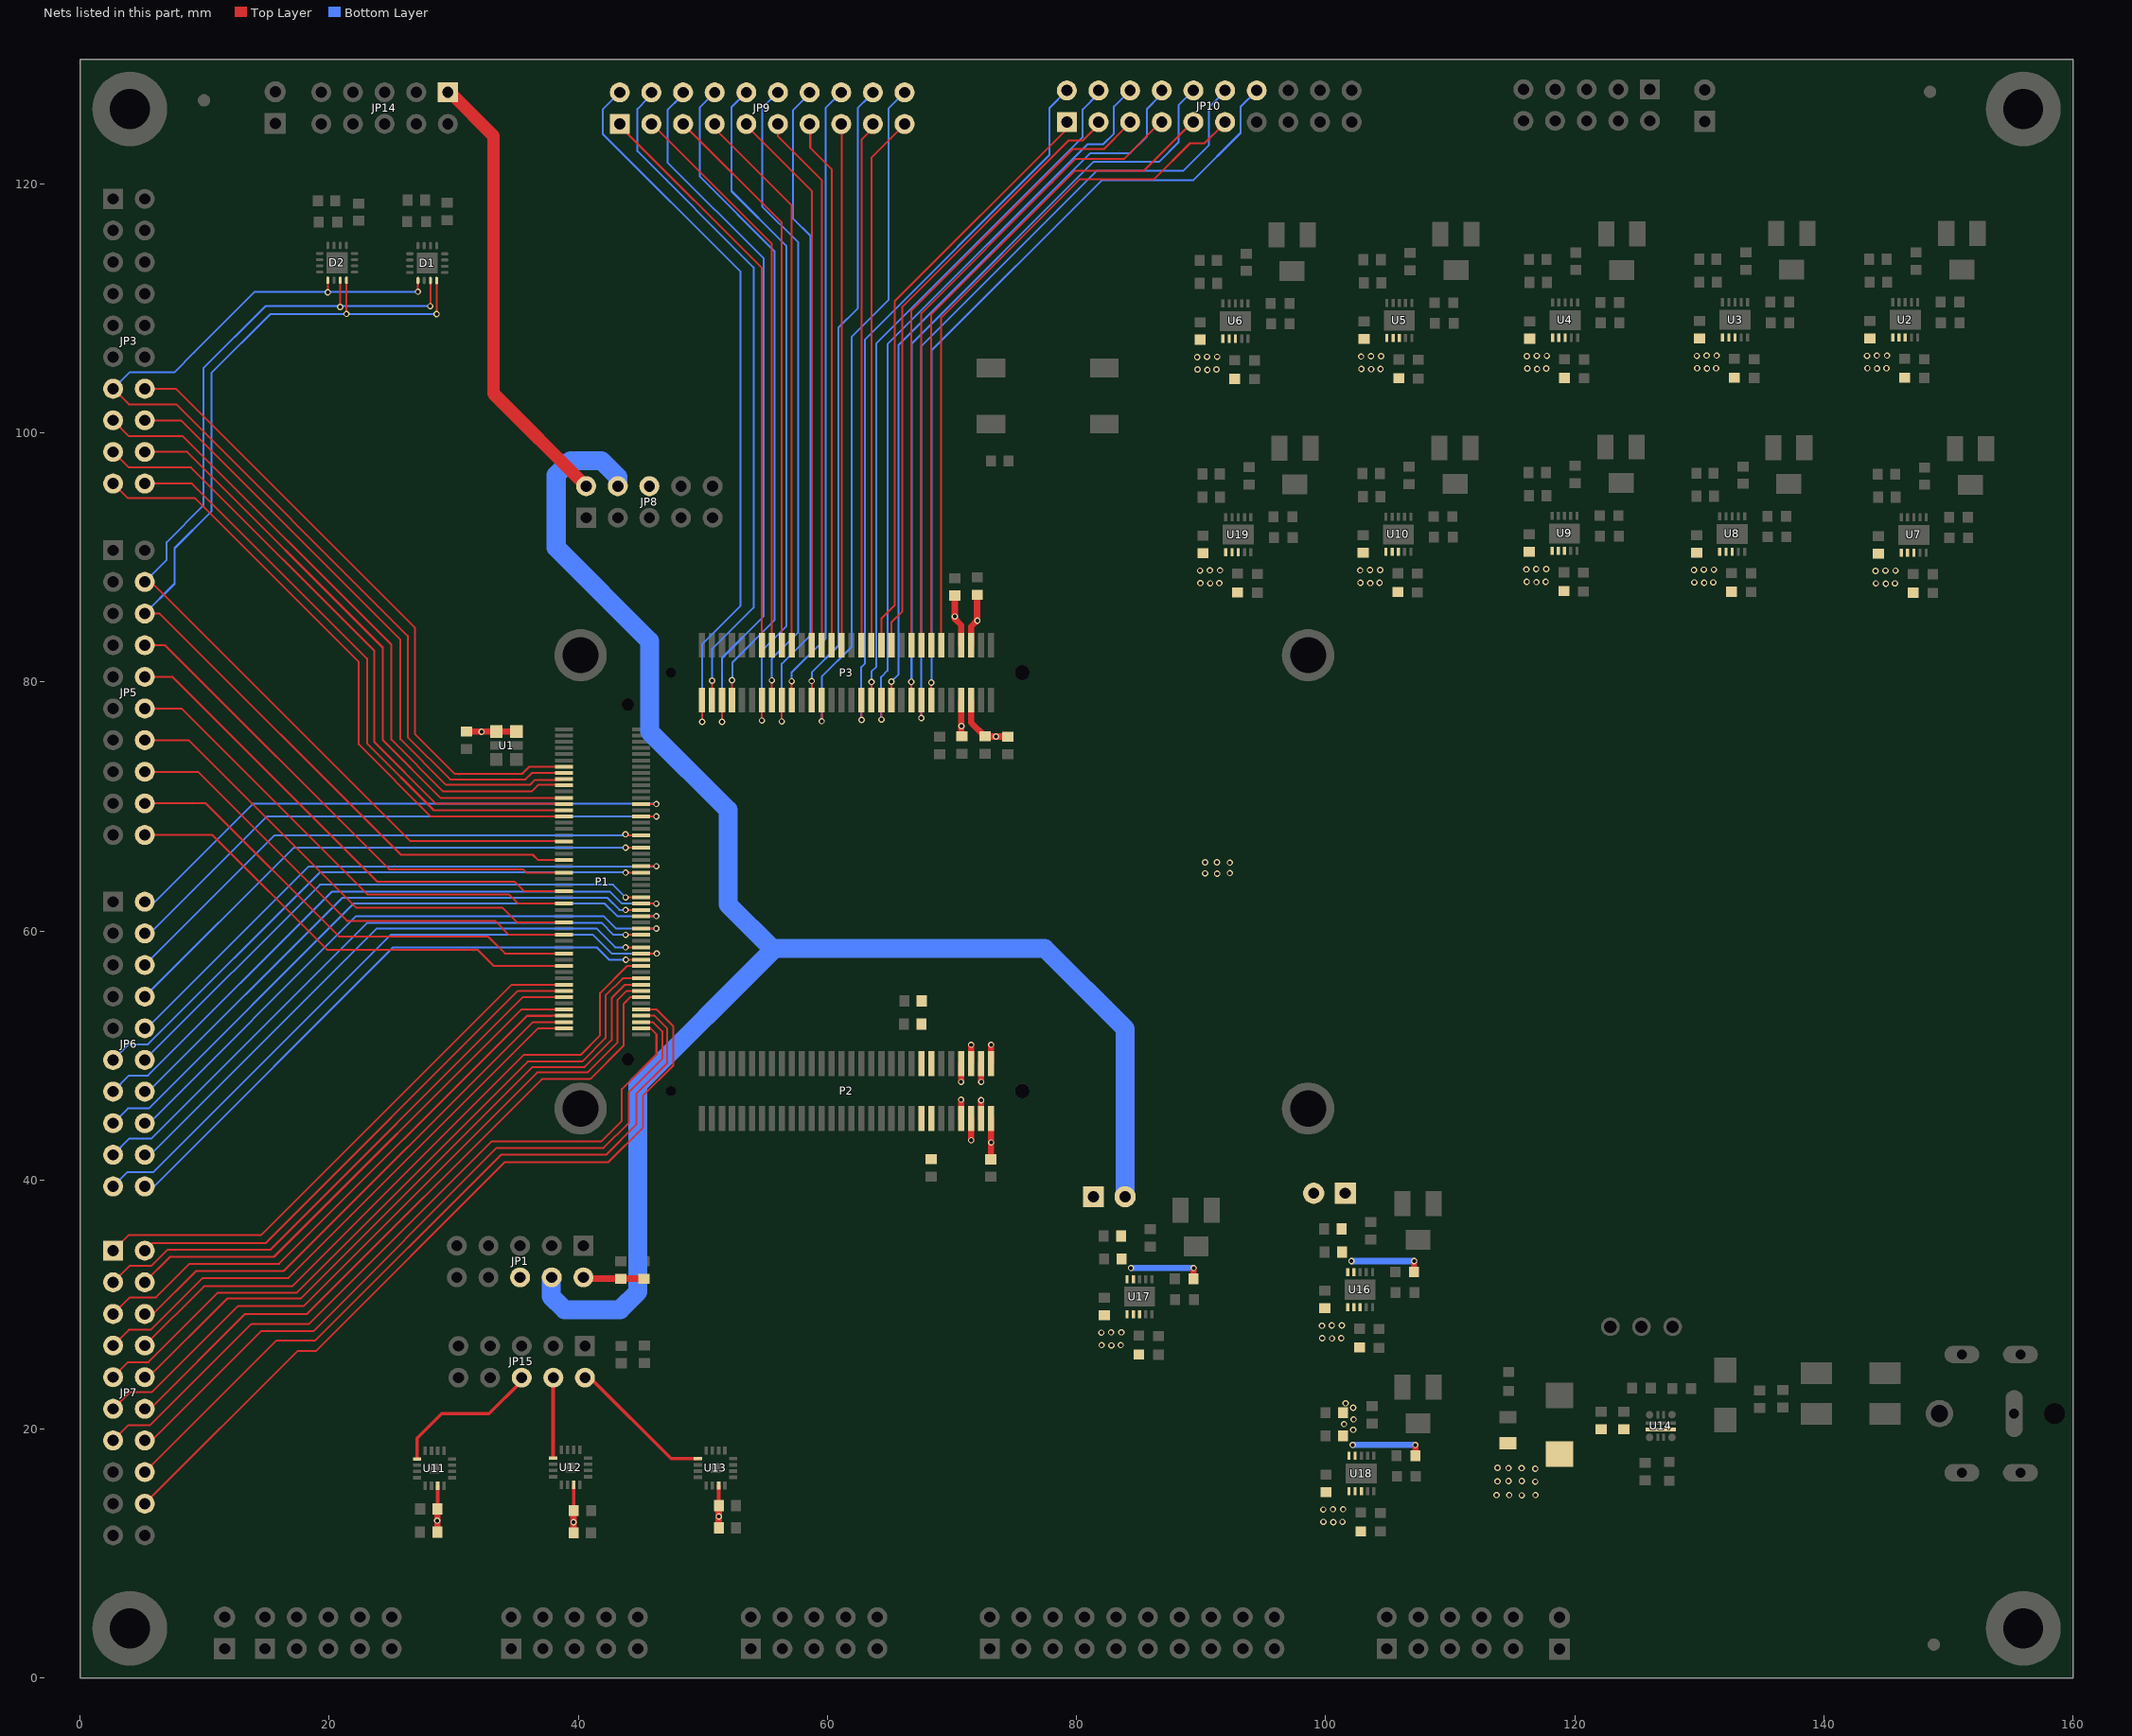
[diagram p0: the nets of this part, all layers, seen from the top]
# Altium PCB MISC82195.PcbDoc (part 6 of 8)
Units mm, origin at the board's own origin, x right, y up, seen from the top; angles counter-clockwise.
Board outline 160 x 130 mm, 4 copper layers (Top Layer, GND, POWER, Bottom Layer); 214 components, 251 nets, 1068 pads, 1218 vias.

## Via types
v1: diameter 0.508, hole 0.305, Top Layer to Bottom Layer, 1218 vias

## Nets (pads, with @x,y where several pads share a name; then routed paths per layer and width w, separated by ;. In a path a pad name is that pad's centre, name@x,y a point inside that pad or via, vN(x,y) a via of type N, cw(c..) or ccw(c..) an arc to the next point about the centre after c; other vN are vias at no path point) (continued)
PW53: JP6.11 P1.B47 | length 48.8
  Top Layer w0.152: v1(43.803,64.688) P1.B47@45.038,64.688
  Bottom Layer w0.152: JP6.11@2.658,49.642 3.918,50.902 5.461,50.902 19.253,64.694 v1@43.965,64.694
PW54: JP6.13 P1.B57 | length 51.9
  Top Layer w0.152: P1.B57@45.038,62.188 v1(46.274,62.188)
  Bottom Layer w0.152: JP6.13@2.658,47.102 3.943,48.387 5.461,48.387 20.244,63.17 42.52,63.17 43.501,62.188 v1(46.274,62.188)
PW55: JP6.15 P1.B61 | length 52.6
  Top Layer w0.152: P1.B61@45.038,61.188 v1(46.274,61.188)
  Bottom Layer w0.152: JP6.15@2.658,44.562 3.841,45.745 5.512,45.745 21.971,62.205 42.113,62.205 43.129,61.188 v1(46.274,61.188)
PW56: JP6.17 P1.B67 | length 50.5
  Top Layer w0.152: v1(43.803,59.688) P1.B67@45.038,59.688
  Bottom Layer w0.152: JP6.17@2.658,42.022 3.968,43.332 5.74,43.332 23.063,60.655 41.859,60.655 42.826,59.688 v1(43.803,59.688)
PW57: JP6.19 P1.B73 | length 53.9
  Top Layer w0.152: P1.B73@45.038,58.188 v1(46.301,58.188)
  Bottom Layer w0.152: JP6.19@2.658,39.482 3.816,40.64 5.893,40.64 24.968,59.715 41.148,59.715 42.672,58.191 46.298,58.191 v1(46.301,58.188)
PW58: JP7.1 P1.B84 | length 45.1
  Top Layer w0.152: JP7.1@2.658,34.326 3.892,35.56 14.529,35.56 34.657,55.688 P1.B84@38.866,55.688
PW59: JP7.3 P1.B88 | length 45.7
  Top Layer w0.152: JP7.3@2.658,31.786 3.968,33.096 5.715,33.096 7.01,34.392 15.265,34.392 35.562,54.688 P1.B88@38.866,54.688
PW60: JP7.5 P1.B94 | length 48.2
  Top Layer w0.152: JP7.5@2.658,29.246 3.994,30.582 6.096,30.582 8.788,33.274 15.977,33.274 35.865,53.162 ; 37.914,53.162 35.865,53.162 ; P1.B94@38.866,53.188 35.891,53.188 35.865,53.162
PW61: JP7.7 P1.B98 | length 46.8
  Top Layer w0.152: JP7.7@2.658,26.706 3.918,27.965 5.69,27.965 9.855,32.131 16.739,32.131 36.796,52.188 P1.B98@38.866,52.188
PW62: JP7.9 P1.B81 | length 58.7
  Top Layer w0.152: JP7.9@2.658,24.166 3.867,25.375 5.486,25.375 11.074,30.963 17.399,30.963 35.941,49.505 40.31,49.505 42.189,51.384 42.189,53.797 ; 42.189,54.331 42.189,53.797 ; 44.086,56.185 43.561,56.185 ; P1.B81@45.038,56.188 43.565,56.188 43.561,56.185 ; 42.189,53.797 42.189,54.813 43.536,56.159 43.561,56.185
PW63: JP7.11 P1.B85 | length 58.3
  Top Layer w0.152: JP7.11@2.658,21.626 3.994,22.962 5.766,22.962 12.675,29.87 17.932,29.87 36.703,48.641 40.742,48.641 43.129,51.029 43.129,54.432 43.885,55.188 P1.B85@45.038,55.188
PW64: JP7.13 P1.B97 | length 61
  Top Layer w0.152: JP7.13@2.658,19.086 3.867,20.295 5.613,20.295 13.767,28.448 18.39,28.448 33.045,43.104 41.859,43.104 43.497,44.742 43.497,47.307 46.279,50.089 46.279,51.689 45.771,52.197 P1.B97@45.441,52.197 ; P1.B97@45.038,52.188 P1.B97@45.441,52.188
PW65: JP7.18 P1.B91 | length 64.8
  Top Layer w0.152: JP7.18@5.198,14.006 17.456,26.264 18.923,26.264 34.087,41.427 42.418,41.427 45.212,44.221 45.212,46.787 47.625,49.2 47.625,52.349 46.279,53.696 P1.B91@45.491,53.696 ; P1.B91@45.038,53.688 P1.B91@45.491,53.688
PW66: JP7.16 P1.B93 | length 62.3
  Top Layer w0.152: JP7.16@5.198,16.546 15.754,27.102 18.872,27.102 33.807,42.037 42.24,42.037 44.653,44.45 44.653,46.914 47.142,49.403 47.142,52.172 46.126,53.188 P1.B93@45.415,53.188 ; P1.B93@45.038,53.188 P1.B93@45.415,53.188
PW67: JP7.14 P1.B95 | length 59.9
  Top Layer w0.152: JP7.14@5.198,19.086 5.751,19.086 14.529,27.864 18.745,27.864 33.452,42.57 42.037,42.57 44.069,44.602 44.069,47.066 46.736,49.733 46.736,51.867 46.736,51.943 45.991,52.688 P1.B95@45.038,52.688
PW68: JP7.12 P1.B87 | length 55.7
  Top Layer w0.152: JP7.12@5.198,21.626 5.624,21.626 13.233,29.235 18.212,29.235 37.084,48.108 40.97,48.108 43.637,50.775 43.637,53.01 ; 43.637,53.213 43.637,53.01 ; P1.B87@44.577,54.686 44.196,54.686 43.637,54.127 43.637,53.01 ; P1.B87@44.577,54.688 P1.B87@45.038,54.688
PW69: JP7.10 P1.B83 | length 55.5
  Top Layer w0.152: JP7.10@5.198,24.166 5.497,24.166 11.811,30.48 17.729,30.48 36.322,49.073 40.513,49.073 42.672,51.232 42.672,53.772 ; 42.672,54.077 42.672,53.772 ; 44.086,55.677 43.739,55.677 ; P1.B83@45.038,55.688 43.75,55.688 43.739,55.677 ; 42.672,53.772 42.672,54.61 43.713,55.651 43.739,55.677
PW70: JP7.8 P1.B77 | length 55
  Top Layer w0.152: JP7.8@5.198,26.706 9.963,31.471 17.043,31.471 35.611,50.038 40.183,50.038 41.758,51.613 41.758,54 ; 41.758,54.508 41.758,54 ; P1.B77@45.038,57.188 43.93,57.188 41.758,55.016 41.758,54
PW71: JP7.6 P1.B96 | length 43.4
  Top Layer w0.152: JP7.6@5.198,29.246 5.878,29.246 9.322,32.69 16.358,32.69 36.356,52.688 P1.B96@38.866,52.688
PW72: JP7.4 P1.B92 | length 42.7
  Top Layer w0.152: JP7.4@5.198,31.786 7.245,33.833 15.57,33.833 35.426,53.688 P1.B92@38.866,53.688
PW73: JP7.2 P1.B86 | length 42.3
  Top Layer w0.152: JP7.2@5.198,34.326 5.797,34.925 14.884,34.925 35.148,55.188 P1.B86@38.866,55.188
PW74: JP6.20 P1.B75 | length 48.2
  Top Layer w0.152: v1(43.82,57.688) P1.B75@45.038,57.688
  Bottom Layer w0.152: JP6.20@5.198,39.482 5.928,39.482 25.121,58.674 41.478,58.674 42.464,57.688 v1(43.82,57.688)
PW75: JP6.18 P1.B71 | length 48
  Top Layer w0.152: v1(43.804,58.688) P1.B71@45.038,58.688
  Bottom Layer w0.152: JP6.18@5.198,42.022 5.649,42.022 23.8,60.173 41.478,60.173 42.962,58.688 v1(43.804,58.688)
PW76: JP6.16 P1.B65 | length 49.6
  Top Layer w0.152: P1.B65@45.038,60.188 v1(46.274,60.188)
  Bottom Layer w0.152: JP6.16@5.198,44.562 5.547,44.562 22.174,61.189 42.037,61.189 43.037,60.188 v1(46.274,60.188)
PW77: JP6.14 P1.B59 | length 46.7
  Top Layer w0.152: v1(43.803,61.688) P1.B59@45.038,61.688
  Bottom Layer w0.152: JP6.14@5.198,47.102 5.497,47.102 21.057,62.662 42.342,62.662 43.315,61.688 v1(43.803,61.688)
PW78: JP6.12 P1.B55 | length 46.1
  Top Layer w0.152: v1(43.803,62.688) P1.B55@45.038,62.688
  Bottom Layer w0.152: JP6.12@5.198,49.642 19.262,63.706 42.786,63.706 v1(43.803,62.688)
PW79: JP6.10 P1.B45 | length 47.7
  Top Layer w0.152: P1.B45@45.038,65.188 v1(46.274,65.188)
  Bottom Layer w0.152: JP6.10@5.198,52.182 5.37,52.182 18.364,65.176 v1@46.262,65.176
PW80: JP6.8 P1.B39 | length 44.8
  Top Layer w0.152: v1(43.803,66.688) P1.B39@45.038,66.688
  Bottom Layer w0.152: JP6.8@5.198,54.722 17.176,66.7 v1@43.79,66.7
PW81: JP6.6 P1.B35 | length 44.3
  Top Layer w0.152: v1(43.79,67.767) 43.79,67.702 43.803,67.688 P1.B35@45.038,67.688
  Bottom Layer w0.152: JP6.6@5.198,57.262 15.627,67.691 v1@43.815,67.691
PW82: JP6.4 P1.B29 | length 46.2
  Top Layer w0.152: P1.B29@45.038,69.188 v1(46.274,69.188)
  Bottom Layer w0.152: JP6.4@5.198,59.802 5.598,59.802 14.986,69.19 46.273,69.19 v1(46.274,69.188)
PW83: JP6.2 P1.B25 | length 46
  Top Layer w0.152: P1.B25@45.038,70.188 v1(46.274,70.188)
  Bottom Layer w0.152: JP6.2@5.198,62.342 6.03,62.342 13.894,70.206 43.485,70.206 ; 43.891,70.206 43.485,70.206 ; v1(46.274,70.188) 46.257,70.206 43.485,70.206
PW84: JP5.20 P1.B78 | length 38
  Top Layer w0.152: JP5.20@5.198,67.701 10.632,67.701 19.837,58.496 31.902,58.496 33.21,57.188 P1.B78@38.866,57.188
PW85: JP5.18 P1.B74 | length 38.3
  Top Layer w0.152: JP5.18@5.198,70.241 10.099,70.241 20.777,59.563 32.741,59.563 34.112,58.191 P1.B74@38.506,58.191
PW86: JP5.16 P1.B68 | length 38.7
  Top Layer w0.152: JP5.16@5.198,72.781 9.464,72.781 21.438,60.808 33.325,60.808 34.442,59.69 P1.B68@38.481,59.69
PW87: JP5.14 P1.B64 | length 39.7
  Top Layer w0.152: JP5.14@5.198,75.321 8.727,75.321 22.174,61.874 33.909,61.874 35.103,60.681 P1.B64@38.837,60.681
PW88: JP5.12 P1.B58 | length 40.2
  Top Layer w0.152: JP5.12@5.198,77.861 8.143,77.861 23.063,62.941 34.442,62.941 35.195,62.188 P1.B58@38.866,62.188
PW89: JP5.10 P1.B54 | length 40.8
  Top Layer w0.152: JP5.10@5.198,80.401 7.407,80.401 23.851,63.957 34.9,63.957 35.668,63.188 P1.B54@38.866,63.188
PW90: JP5.8 P1.B48 | length 41.2
  Top Layer w0.152: JP5.8@5.198,82.941 6.822,82.941 24.816,64.948 35.56,64.948 35.819,64.688 P1.B48@38.866,64.688
PW91: D1.8 D2.8 JP5.6 P1.B44 | length 88.7
  Top Layer w0.152: JP5.6@5.198,85.481 6.391,85.481 25.756,66.116 36.347,66.116 36.775,65.688 P1.B44@38.866,65.688 ; v1(21.391,109.546) D2.8@21.391,112.25 ; v1@28.63,109.707 D1.8@28.63,112.224
  Bottom Layer w0.152: JP5.6@5.198,85.481 7.595,87.878 7.595,90.729 10.566,93.701 10.566,104.826 15.265,109.525 v1(28.626,109.525)
PW92: D1.7 D2.7 JP5.4 P1.B38 | length 86.2
  Top Layer w0.152: JP5.4@5.198,88.021 5.73,88.021 26.543,67.208 37.262,67.208 ; v1(20.891,110.096) D2.7@20.891,112.25 ; v1@28.13,110.248 D1.7@28.13,112.224 ; 37.897,67.208 37.262,67.208 ; P1.B38@38.608,67.208 37.262,67.208
  Bottom Layer w0.152: JP5.4@5.198,88.021 6.96,89.783 6.96,89.916 6.96,91.211 9.906,94.158 9.906,105.181 14.884,110.16 v1(28.118,110.16)
PW94: D1.5 D2.5 JP3.13 P1.B16 | length 83.7
  Top Layer w0.152: JP3.13@2.658,103.541 3.913,102.286 7.722,102.286 26.314,83.693 26.314,75.565 29.718,72.161 35.763,72.161 36.29,72.688 P1.B16@38.866,72.688 ; v1(19.891,111.28) D2.5@19.891,112.25 ; v1@27.13,111.407 D1.5@27.13,112.224
  Bottom Layer w0.152: JP3.13@2.658,103.541 3.968,104.851 7.569,104.851 9.182,106.464 14.046,111.328 v1(27.127,111.328)
PW95: JP3.14 P1.B14 | length 51.7
  Top Layer w0.152: JP3.14@5.198,103.541 7.686,103.541 26.873,84.353 26.873,75.819 30.074,72.619 35.509,72.619 36.079,73.188 P1.B14@38.866,73.188
PW96: JP3.15 P1.B20 | length 52.7
  Top Layer w0.152: JP3.15@2.658,101.001 3.938,99.72 8.255,99.72 24.994,82.982 24.994,75.362 29.159,71.196 36.246,71.196 36.779,71.73 P1.B20@38.354,71.73
PW97: JP3.16 P1.B18 | length 50.4
  Top Layer w0.152: JP3.16@5.198,101.001 8.118,101.001 25.73,83.388 25.73,75.387 29.388,71.73 36.119,71.73 36.525,72.136 P1.B18@38.608,72.136
PW98: JP3.17 P1.B26 | length 52.3
  Top Layer w0.152: JP3.17@2.658,98.461 3.913,97.206 8.915,97.206 23.622,82.499 23.622,75.159 28.575,70.206 37.592,70.206 ; 37.914,70.206 37.592,70.206 ; P1.B26@38.583,70.206 37.592,70.206
PW99: JP3.18 P1.B24 | length 49.1
  Top Layer w0.152: JP3.18@5.198,98.461 8.6,98.461 24.308,82.753 24.308,75.311 28.956,70.663 P1.B24@38.405,70.663
PW100: JP3.19 P1.B30 | length 50.9
  Top Layer w0.152: JP3.19@2.658,95.921 3.836,94.742 9.246,94.742 22.377,81.61 22.377,74.981 28.169,69.19 37.668,69.19 ; 37.871,69.19 37.668,69.19 ; P1.B30@38.43,69.19 37.668,69.19
PW101: JP3.20 P1.B28 | length 48.5
  Top Layer w0.152: JP3.20@5.198,95.921 8.981,95.921 23.038,81.864 23.038,75.057 28.406,69.688 P1.B28@38.866,69.688
PW102: JP9.1 P3.C13 | length 45.5
  Top Layer w0.152: JP9.1@43.967,124.003 54.737,113.233 P3.C13@54.737,82.939
PW103: JP9.3 P3.C15 | length 45.1
  Top Layer w0.152: JP9.3@46.431,124.282 55.537,115.176 P3.C15@55.537,82.939
PW104: JP9.5 P3.C17 | length 44.7
  Top Layer w0.152: JP9.5@48.692,124.511 56.337,116.865 P3.C17@56.337,82.939
PW105: JP9.7 P3.C19 | length 43.7
  Top Layer w0.152: JP9.7@51.181,124.206 57.137,118.25 P3.C19@57.137,82.939
PW106: JP9.9 P3.C23 | length 43.4
  Top Layer w0.152: JP9.9@53.873,124.282 58.737,119.418 P3.C23@58.737,82.939
PW107: JP9.11 P3.C25 | length 42.9
  Top Layer w0.152: JP9.11@56.007,124.384 56.007,123.825 59.537,120.295 P3.C25@59.537,82.939
PW108: JP9.13 P3.C27 | length 42.2
  Top Layer w0.152: JP9.13@58.623,124.409 58.623,122.885 60.337,121.171 P3.C27@60.337,82.939
PW109: JP9.15 P3.C29 | length 41.4
  Top Layer w0.152: P3.C29@61.137,82.939 JP9.15@61.137,124.359
PW110: JP9.17 P3.C33 | length 42
  Top Layer w0.152: P3.C33@62.737,82.939 62.737,123.52 JP9.17@63.754,124.536
PW111: JP9.19 P3.C35 | length 42.7
  Top Layer w0.152: P3.C35@63.537,82.939 63.537,122.084 JP9.19@66.04,124.587
PW112: JP10.1 P3.C37 | length 47.6
  Top Layer w0.152: P3.C37@64.337,82.939 64.337,85.089 65.405,86.157 65.405,110.566 JP10.1@79.248,124.409
PW113: JP10.3 P3.C39 | length 49.2
  Top Layer w0.152: P3.C39@65.137,82.939 65.137,84.797 66.015,85.674 66.015,110.134 79.35,123.469 80.493,123.469 JP10.3@81.661,124.638
PW114: JP10.5 P3.C43 | length 50.2
  Top Layer w0.152: P3.C43@66.737,82.939 66.737,109.816 77.673,120.752 77.749,120.828 79.705,122.784 82.22,122.784 JP10.5@83.972,124.536
PW115: JP10.7 P3.C45 | length 51.3
  Top Layer w0.152: P3.C45@67.539,83.617 67.539,109.601 78.003,120.066 78.08,120.142 79.908,121.971 83.795,121.971 JP10.7@86.589,124.765
PW116: JP10.9 P3.C47 | length 53.8
  Top Layer w0.152: P3.C47@68.337,82.939 68.337,109.511 79.883,121.056 85.42,121.056 JP10.9@89.027,124.663 ; JP10.9@89.052,124.638 JP10.9@89.205,124.79
PW117: JP10.11 P3.C49 | length 54.6
  Top Layer w0.152: P3.C49@69.139,83.566 69.139,109.245 80.264,120.371 86.233,120.371 89.103,123.241 90.272,123.241 JP10.11@91.669,124.638 ; JP10.11@91.707,124.6 JP10.11@91.745,124.638
PW118: JP10.14 P3.C48 | length 64
  Top Layer w0.152: P3.C48@68.337,78.539 v1(68.337,79.945)
  Bottom Layer w0.152: v1@68.351,80.01 68.351,106.604 82.017,120.269 89.357,120.269 93.167,124.079 93.167,126.187 JP10.14@94.463,127.483
PW119: JP10.12 P3.C46 | length 65.7
  Top Layer w0.152: v1(67.537,77.09) P3.C46@67.537,78.539
  Bottom Layer w0.152: v1(67.537,77.09) 67.537,106.958 81.61,121.031 88.544,121.031 90.627,123.114 90.627,126.136 JP10.12@91.745,127.254
PW120: JP10.10 P3.C44 | length 61.3
  Top Layer w0.152: P3.C44@66.737,78.539 v1(66.737,79.998)
  Bottom Layer w0.152: v1@66.751,80.086 66.751,107.137 81.382,121.768 86.639,121.768 88.189,123.317 88.189,126.289 JP10.10@89.383,127.483
PW121: JP10.8 P3.C40 | length 59.3
  Top Layer w0.152: P3.C40@65.137,78.539 v1(65.137,80.022)
  Bottom Layer w0.152: v1(65.137,80.022) 65.71,80.594 65.71,107.061 81.102,122.453 84.303,122.453 85.649,123.8 85.649,126.009 JP10.8@86.69,127.051
PW122: JP10.6 P3.C38 | length 61
  Top Layer w0.152: v1(64.337,76.961) P3.C38@64.337,78.539
  Bottom Layer w0.152: v1@64.313,77.089 64.313,80.391 64.821,80.899 64.821,107.112 80.874,123.165 82.144,123.165 83.007,124.028 83.007,126.187 JP10.6@84.303,127.483
PW123: JP10.4 P3.C36 | length 56.1
  Top Layer w0.152: P3.C36@63.537,78.539 v1(63.537,79.997)
  Bottom Layer w0.152: v1(63.537,79.997) 63.537,80.835 63.932,81.229 63.932,107.188 80.493,123.749 80.493,125.959 JP10.4@81.686,127.152
PW124: JP10.2 P3.C34 | length 58.8
  Top Layer w0.152: v1(62.737,76.937) P3.C34@62.737,78.539
  Bottom Layer w0.152: v1@62.713,77.089 62.713,81.178 63.017,81.483 63.017,107.493 77.826,122.301 77.826,126.086 JP10.2@79.223,127.483
PW125: JP9.20 P3.C26 | length 54.8
  Top Layer w0.152: v1(59.537,76.835) P3.C26@59.537,78.539
  Bottom Layer w0.152: v1@59.563,76.962 59.563,80.442 61.951,82.829 61.951,107.721 64.922,110.693 64.922,126.06 JP9.20@66.192,127.33
PW126: JP9.18 P3.C24 | length 50.3
  Top Layer w0.152: P3.C24@58.737,78.539 v1(58.737,80.073)
  Bottom Layer w0.152: v1(58.737,80.073) 58.737,80.759 60.884,82.906 60.884,108.433 62.433,109.982 62.433,126.06 JP9.18@63.297,126.924
PW127: JP9.16 P3.C20 | length 50.3
  Top Layer w0.152: P3.C20@57.137,78.539 v1(57.137,80.048)
  Bottom Layer w0.152: v1@57.125,80.213 57.125,80.747 59.842,83.464 59.842,126.06 JP9.16@61.112,127.33
PW128: JP9.14 P3.C18 | length 53.8
  Top Layer w0.152: v1(56.337,76.81) P3.C18@56.337,78.539
  Bottom Layer w0.152: v1(56.337,76.81) 56.337,81.102 ; 56.337,81.001 56.337,81.458 58.649,83.769 58.649,115.799 57.252,117.196 57.252,125.908 JP9.14@58.217,126.873
PW129: JP9.12 P3.C16 | length 51
  Top Layer w0.152: P3.C16@55.537,78.539 v1(55.537,80.125)
  Bottom Layer w0.152: v1(55.537,80.125) 55.537,81.877 57.658,83.998 57.658,115.291 54.762,118.186 54.762,126.06 JP9.12@55.753,127.051
PW130: JP9.10 P3.C14 | length 55.1
  Top Layer w0.152: v1(54.737,76.886) P3.C14@54.737,78.539
  Bottom Layer w0.152: JP9.10@53.492,127.33 52.299,126.136 52.299,119.405 56.693,115.011 56.693,84.455 54.712,82.474 v1@54.712,76.987
PW131: JP9.8 P3.C8 | length 53.1
  Top Layer w0.152: P3.C8@52.337,78.539 v1(52.337,80.125)
  Bottom Layer w0.152: JP9.8@50.952,127.33 49.759,126.136 49.759,120.574 55.753,114.579 55.753,84.938 52.375,81.559 v1@52.375,80.213
PW132: JP9.6 P3.C6 | length 56.9
  Top Layer w0.152: v1(51.537,76.785) P3.C6@51.537,78.539
  Bottom Layer w0.152: JP9.6@48.184,126.924 47.168,125.908 47.168,121.717 54.889,113.995 54.889,85.268 51.537,81.916 v1(51.537,76.785)
PW133: JP9.4 P3.C4 | length 53.9
  Top Layer w0.152: P3.C4@50.737,78.539 v1(50.737,80.1)
  Bottom Layer w0.152: JP9.4@45.568,126.822 44.755,126.009 44.755,122.606 54.077,113.284 54.077,85.954 50.737,82.614 v1(50.737,80.1)
PW134: JP9.2 P3.C2 | length 58.6
  Top Layer w0.152: v1(49.937,76.785) P3.C2@49.937,78.539
  Bottom Layer w0.152: JP9.2@43.332,127.33 41.961,125.959 41.961,124.003 53.01,112.954 53.01,86.081 49.936,83.007 v1@49.936,76.937
REF_BL: JP15.4 U12.1 | length 6.1
  Top Layer w0.279: U12.1@37.979,17.677 JP15.4@37.979,23.794
REF_SL: JP15.2 U13.1 | length 11.1
  Top Layer w0.279: JP15.2@41.097,23.978 47.449,17.626 U13.1@49.612,17.626
REF_WL: JP15.6 U11.1 | length 11.9
  Top Layer w0.279: U11.1@27.057,17.6 27.057,19.259 29.032,21.234 32.842,21.234 JP15.6@35.382,23.774
VCC1V8D: C2.2 C3.2 C9.2 C10.2 C11.2 C55.2 C56.2 C75.2 C76.2 JP1.2 JP8.2 JP14.1 JP22.1 P3.C53 P3.C54 P3.C55 P3.C56 R45.2 U18.9 U18.10 | length 62.8
  Top Layer w0.508: JP14.1@29.531,127.34 JP14.1@29.744,127.128 ; JP1.2@40.741,32.081 C56.2@43.418,32.081 C55.2@45.272,32.081 ; v1(70.231,85.242) v1@70.231,85.065 ; C11.2@70.231,86.766 v1@70.231,85.065 ; C9.2@70.737,75.716 v1@70.737,76.454 ; P3.C54@70.737,78.539 v1@70.737,76.454 ; P3.C53@70.737,82.939 70.737,84.558 v1@70.231,85.065 ; v1(70.764,76.454) v1@70.737,76.454 ; P3.C56@71.537,78.539 71.537,76.722 72.644,75.616 v1(73.533,75.616) C3.2@74.27,75.616 ; P3.C55@71.537,82.939 71.537,84.441 v1@72.009,84.912 ; C10.2@72.009,86.766 v1@72.009,84.912 ; v1(72.034,84.912) v1@72.009,84.912 ; R45.2@107.197,17.856 v1(107.197,18.729)
  Top Layer w1.016: JP14.1@29.82,127.203 33.198,123.825 33.198,103.15 JP8.2@40.631,95.717
  Bottom Layer w0.508: v1(102.175,18.729) v1(107.197,18.729)
  other v1: 102.21,19.939 101.473,20.396 102.235,20.777 102.21,21.717 101.6,22.073
VCC2V5D: C72.2 C73.2 JP1.4 JP8.4 JP22.2 R44.2 U17.9 U17.10 | length 143.7
  Top Layer w0.508: R44.2@89.392,32.055 v1(89.392,32.927)
  Bottom Layer w0.508: v1(84.37,32.927) v1(89.392,32.927)
  Bottom Layer w1.524: JP1.4@37.821,32.207 37.821,30.658 38.887,29.591 43.358,29.591 44.78,31.013 44.78,47.625 55.651,58.496 52.019,62.128 52.019,69.723 45.72,76.022 45.72,83.287 38.227,90.78 38.227,96.622 39.37,97.765 41.859,97.765 43.18,96.444 JP8.4@43.18,95.809 ; 55.753,58.598 77.445,58.598 83.896,52.146 JP22.2@83.896,38.659
VCC3V3D: C1.1 C4.2 C5.2 C6.2 C69.2 C70.2 JP1.6 JP8.6 JP19.1 P2.A45 P2.A46 P2.A47 P2.A48 R43.2 U1.1 U1.6 U16.9 U16.10 | length 9.6
  Top Layer w0.508: C1.1@31.387,76.014 v1@32.233,76.014 ; v1(32.233,75.997) v1@32.233,76.014 ; U1.6@35.03,76.014 U1.1@33.43,76.014 v1@32.233,76.014 ; R43.2@107.095,32.614 v1(107.095,33.486)
  Bottom Layer w0.508: v1(102.074,33.486) v1(107.095,33.486)
  other v1: 91.288,64.592 90.322,64.618 92.304,64.643 92.304,65.481 90.322,65.507 91.262,65.507
VCC5VD: C7.2 C13.2 C16.2 C19.2 C25.2 C28.2 C31.2 C37.2 C40.2 C43.2 C49.2 C50.2 C51.2 C52.2 C53.2 C54.2 C63.2 C64.2 C68.2 C71.2 C74.2 C80.2 D3.1 JP19.2 LED1.1 P2.A53 P2.A54 P2.A55 P2.A56 P2.A57 P2.A58 P2.A59 P2.A60 R4.2 R5.2 R6.2 R16.2 R17.2 R18.2 R28.2 R29.2 R30.2 R46.2 R47.2 R48.2 R56.2 U2.1 U2.2 U2.3 U3.1 U3.2 U3.3 U4.1 U4.2 U4.3 U5.1 U5.2 U5.3 U6.1 U6.2 U6.3 U7.1 U7.2 U7.3 U8.1 U8.2 U8.3 U9.1 U9.2 U9.3 U10.1 U10.2 U10.3 U11.7 U12.7 U13.7 U14.6 U16.1 U16.2 U16.3 U17.1 U17.2 U17.3 U18.1 U18.2 U18.3 U19.1 U19.2 U19.3 | length 23.4
  Top Layer w0.279: C49.2@28.714,13.754 U11.7@28.714,15.443 ; C51.2@39.636,13.703 U12.7@39.636,15.519 ; C54.2@51.269,14.033 U13.7@51.269,15.468
  Top Layer w0.508: v1(28.677,12.649) v1@28.682,12.649 ; C50.2@28.682,11.72 v1@28.682,12.649 ; C49.2@28.682,13.264 v1@28.682,12.649 ; C52.2@39.619,11.674 v1@39.619,12.522 ; C51.2@39.619,13.467 v1@39.619,12.522 ; v1(39.624,12.522) v1@39.619,12.522 ; C53.2@51.278,12.08 v1@51.278,12.979 ; C54.2@51.278,13.432 v1@51.278,12.979 ; v1(51.283,12.979) v1@51.278,12.979 ; P2.A54@70.737,44.938 v1(70.737,46.455) ; v1(70.737,47.877) P2.A53@70.737,49.338 ; v1(71.537,43.194) P2.A56@71.537,44.938 ; P2.A55@71.537,49.338 v1(71.537,50.862) ; P2.A58@72.337,44.938 v1(72.337,46.404) ; v1(72.337,47.877) P2.A57@72.337,49.338 ; C7.2@73.137,41.895 v1@73.137,43.002 ; v1(73.137,43.013) v1@73.137,43.002 ; P2.A60@73.137,44.938 v1@73.137,43.002 ; P2.A59@73.137,49.338 v1(73.137,50.862)
  other v1: 100.609,12.522 99.822,12.548 101.346,12.548 99.797,13.538 100.584,13.564 101.397,13.564 115.748,14.681 113.716,14.707 114.732,14.707 116.84,14.707 116.815,15.773 113.792,15.799 114.681,15.824 115.748,15.824 116.815,16.815 114.681,16.866 115.722,16.866 113.792,16.891 82.804,26.721 82.017,26.746 83.541,26.746 100.508,27.28 99.72,27.305 101.244,27.305 81.991,27.737 82.779,27.762 83.591,27.762 99.695,28.296 100.482,28.321 101.295,28.321 144.958,87.884 90.729,87.909 144.17,87.909 145.694,87.909 89.941,87.935 91.465,87.935 103.581,87.935 102.794,87.96 104.318,87.96 130.378,87.96 129.591,87.986 131.115,87.986 116.916,88.011 116.129,88.036 117.653,88.036 144.145,88.9 89.916,88.925 144.932,88.925 145.745,88.925 90.703,88.951 91.516,88.951 102.768,88.951 103.556,88.976 104.369,88.976 129.565,88.976 130.353,89.002 131.166,89.002 116.103,89.027 116.891,89.052 117.704,89.052 90.5,105.054 89.713,105.08 91.237,105.08 103.657,105.105 102.87,105.131 104.394,105.131 116.967,105.131 116.18,105.156 117.704,105.156 130.607,105.156 144.272,105.156 129.819,105.181 131.343,105.181 143.485,105.181 145.009,105.181 89.687,106.07 90.475,106.096 91.288,106.096 102.845,106.121 103.632,106.147 104.445,106.147 116.154,106.147 116.942,106.172 117.754,106.172 129.794,106.172 143.459,106.172 130.581,106.197 131.394,106.197 144.247,106.197 145.059,106.197
pads on no net: D1.1 D1.3 D1.4 D1.9 D1.10 D1.12 D2.1 D2.3 D2.4 D2.9 D2.10 D2.12 F1.1 F2.1 F3.1 F4.1 JP1.8 JP1.10 JP8.8 JP8.10 M1.1 M2.1 M3.1 M4.1 P1. P2. P2.A35 P2.A37 P2.A39 P2.A41 P3. P3.C60 SW1.1 U1.2 U14.2 U14.3 U14.4 U14.10 U15.0 VR1.1 VR2.1 VR3.1 VR4.1 VR5.1 VR6.1 VR7.1 VR8.1 VR9.1 VR10.1 VR11.1 VR12.1 VR13.1
copper on no net:
  other v1: 99.085,21.311

## Polygon pours and split planes (outlines as drawn)
GND on Top Layer "Bottom Layer-No Net" (solid, remove dead copper, pour order 1033): -4.039,124.394 -4.039,-0.65 -0.305,-4.384 1.549,-6.238 6.477,-6.238 165.659,-6.238 167.894,-4.003 170.891,-1.006 170.891,2.398 170.891,134.528 170.129,135.29 163.754,141.666 146.863,141.666 3.835,141.666 -1.422,136.408 -4.42,133.411 -4.42,126.273
VCC3V3D on Top Layer "Bottom Layer-No Net" (solid, remove dead copper, pour order 1032): 67.132,54.178 67.132,50.724 67.158,50.698 67.285,50.571 67.285,50.394 67.285,41.631 67.589,41.326 67.64,41.275 68.021,41.275 68.732,41.275 68.809,41.351 68.834,41.377 68.859,41.377 68.859,42.443 68.732,42.57 68.58,42.723 68.58,44.526 68.58,51.308 69.088,51.816 71.857,54.585 75.311,54.585 87.452,54.585 91.846,58.979 93.98,61.112 93.98,63.983 93.98,64.795 93.345,65.43 92.837,65.938 91.465,65.938 89.789,65.938 88.9,65.049 82.956,59.106 79.883,59.106 70.637,59.106 67.564,56.032 67.132,55.601 67.132,54.204